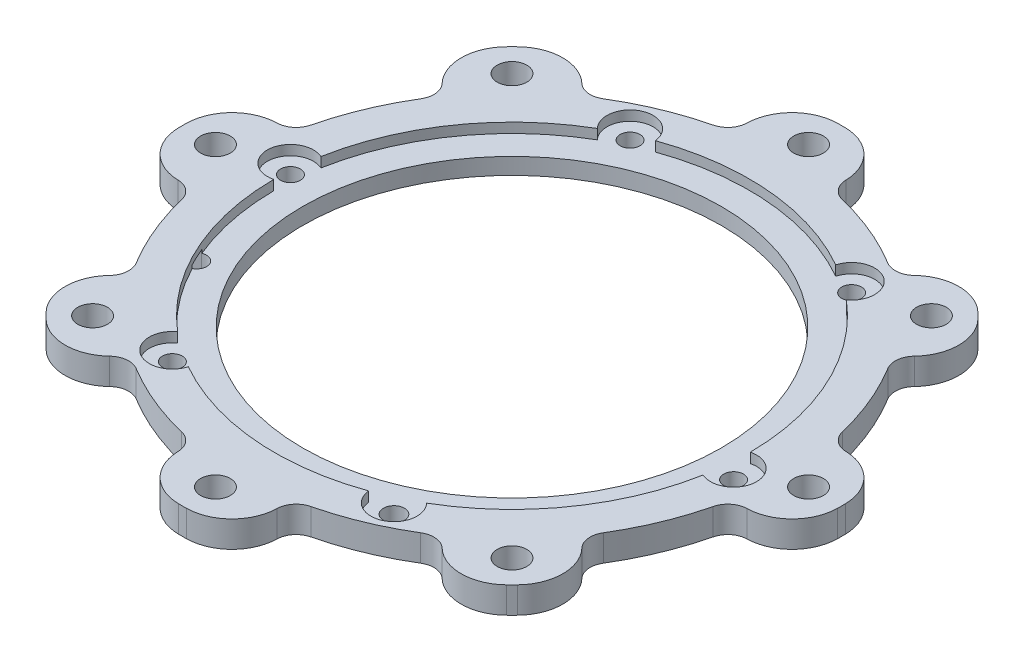
SolidWorks part; units mm, degrees
material "7075-T6 (SN)"
ref_plane "Front Plane" through (0, 0, 0) normal (0, 0, 1) x (1, 0, 0)
ref_plane "Top Plane" through (0, 0, 0) normal (0, 1, 0) x (1, 0, 0)
ref_plane "Right Plane" through (0, 0, 0) normal (1, 0, 0) x (0, 0, -1)
sketch "Sketch1" plane through (0, 0, 0) normal (0, 1, 0) x (1, 0, 0)
  circle A0 centre (0, 0) radius 50
  circle A1 centre (0, 0) radius 30
  dimension "D1" = 100
  dimension "D2" = 60
extrude "Boss-Extrude1" add sketch "Sketch1" along normal blind 4
sketch "Sketch2" plane through (0, 4, 0) normal (0, 1, 0) x (1, 0, 0)
  circle A0 centre (0, 0) radius 39
  circle A1 centre (0, 0) radius 30
  circle A2 centre (0, 0) radius 30 construction
  dimension "D1" = 78
extrude "Boss-Extrude2" add sketch "Sketch2" along normal blind 1
sketch "Sketch3" plane through (0, 0, 0) normal (0, -1, 0) x (1, 0, 0)
  circle A0 centre (0, 0) radius 31.75
  dimension "D1" = 63.5
extrude "Cut-Extrude1" cut sketch "Sketch3" against normal blind 1
sketch "Sketch4" plane through (0, 0, 0) normal (0, -1, 0) x (1, 0, 0)
  line L0 (0, 0) -> (50000, 0) construction
  line L1 (0, 0) -> (0, 50000) construction
  circle A0 centre (0, 0) radius 45 construction
  circle A1 centre (0, 45) radius 2.25
  dimension "D1" = 90
  dimension "D2" = 4.5
extrude "Cut-Extrude2" cut sketch "Sketch4" against normal blind 10
pattern_circular "CirPattern1" count 8 over 360 about axis through (0, 0, 0) along (0, 1, 0) of "Cut-Extrude2"
sketch "Sketch5" plane through (0, 0, 0) normal (0, -1, 0) x (1, 0, 0)
  circle A0 centre (0, 0) radius 31.75 construction
  circle A1 centre (0, 0) radius 31.75
extrude "Cut-Extrude3" cut sketch "Sketch5" against normal blind 27
sketch "Sketch6" plane through (0, 5, 0) normal (0, 1, 0) x (1, 0, 0)
  line L0 (0, 0) -> (49808.2107, -4375.1737) construction
  line L1 (0, 50) -> (0, -49950) construction
  line L2 (0, 0) -> (-50000, 0) construction
  circle A0 centre (0, 0) radius 37 construction
  circle A1 centre (36.8581, -3.2376) radius 3.5
  dimension "D1" = 74
  dimension "D2" = 7
  dimension "D3" = 84.98
extrude "Cut-Extrude4" cut sketch "Sketch6" against normal blind 2.5
pattern_circular "CirPattern2" count 6 over 360 about axis through (0, 0, 0) along (0, 1, 0) of "Cut-Extrude4"
sketch "Sketch7" plane through (0, 5, 0) normal (0, 1, 0) x (1, 0, 0)
  circle A0 centre (-21.2329, -30.3012) radius 1.5
  circle A1 centre (15.6252, -33.5388) radius 1.5978
  circle A2 centre (36.8581, -3.2376) radius 1.5
  circle A3 centre (21.2329, 30.3012) radius 1.5
  circle A4 centre (-15.6252, 33.5388) radius 1.5
  circle A5 centre (-36.8581, 3.2376) radius 1.5
  dimension "D1" = 3
extrude "Cut-Extrude5" cut sketch "Sketch7" against normal blind 15
sketch "Sketch8" plane through (0, 0, 0) normal (0, -1, 0) x (1, 0, 0)
  line L0 (0, 0) -> (50000, 0) construction
  line L1 (0, 0) -> (0, 50000) construction
  line L2 (0, 0) -> (20734.6621, -45498.0635) construction
  line L3 (0, 0) -> (35355.3391, -35355.3391) construction
  line L4 (7.5, -40.8167) -> (7.5, -49.4343)
  line L5 (23.5584, -34.165) -> (29.652, -40.2586)
  circle A2 centre (0, 0) radius 50 construction
  arc A3 (7.5, -40.8167) -> (23.5584, -34.165) centre (0, 0) ccw
  arc A4 (7.5, -49.4343) -> (29.652, -40.2586) centre (0, 0) ccw
  dimension "D4" = 41.5
  dimension "D1" = 24.5
  dimension "D2" = 15
  dimension "D3" = 15
extrude "Cut-Extrude6" cut sketch "Sketch8" against normal blind 13
pattern_circular "CirPattern3" count 8 over 360 about axis through (0, 0, 0) along (0, 1, 0) of "Cut-Extrude6"
fillet "Fillet1" radius 3 16 edges at (-7.5, 2, -40.8167) (-23.5584, 2, -34.165) (-34.165, 2, -23.5584) (-40.8167, 2, -7.5) (-40.8167, 2, 7.5) (-34.165, 2, 23.5584) (-23.5584, 2, 34.165) (-7.5, 2, 40.8167) (7.5, 2, 40.8167) (23.5584, 2, 34.165) (34.165, 2, 23.5584) (40.8167, 2, 7.5) (40.8167, 2, -7.5) (34.165, 2, -23.5584) (23.5584, 2, -34.165) (7.5, 2, -40.8167)
sketch "Sketch9" plane through (0, 5, 0) normal (0, 1, 0) x (1, 0, 0)
  circle A0 centre (0, 0) radius 36
  dimension "D1" = 72
extrude "Cut-Extrude7" cut sketch "Sketch9" against normal up to surface (2.5 mm away) up to face at (-15.6252, 2.5, -32.0388)
fillet "Fillet2" radius 7 16 edges at (40.2586, 2, -29.652) (29.652, 2, -40.2586) (7.5, 2, -49.4343) (-7.5, 2, -49.4343) (-29.652, 2, -40.2586) (-40.2586, 2, -29.652) (-49.4343, 2, -7.5) (-49.4343, 2, 7.5) (-40.2586, 2, 29.652) (-29.652, 2, 40.2586) (-7.5, 2, 49.4343) (7.5, 2, 49.4343) (29.652, 2, 40.2586) (40.2586, 2, 29.652) (49.4343, 2, 7.5) (49.4343, 2, -7.5)
sketch "Sketch10" plane through (0, 5, 0) normal (0, 1, 0) x (1, 0, 0)
  circle A0 centre (0, 0) radius 50
  dimension "D1" = 100
extrude "Cut-Extrude8" cut sketch "Sketch10" against normal up to surface (1 mm away) up to face at (0, 4, 0)
sketch "Sketch12" plane through (0, 0, 0) normal (0, -1, 0) x (1, 0, 0)
  line L0 (0, 0) -> (50000, 0) construction
  line L1 (0, 0) -> (-45322.7627, 21115.0937) construction
  line L2 (-36.8581, -3.2376) -> (49771.3526, 4371.9361) construction
  circle A0 centre (0, 0) radius 37 construction
  circle A1 centre (-33.5388, 15.6252) radius 1.5
  circle A2 centre (33.5388, -15.6252) radius 1.5
  dimension "D2" = 3
  dimension "D1" = 30
extrude "Cut-Extrude9" cut sketch "Sketch12" against normal blind 3
sketch "Sketch13" plane through (0, 0, 0) normal (0, -1, 0) x (1, 0, 0)
  line L0 (-33.5388, 15.6252) -> (45289.2238, -21099.4686) construction
  line L1 (0, 0) -> (-21115.0937, -45322.7627) construction
  line L2 (-32.6324, 15.2029) -> (-34.4453, 16.0475) construction
  line L3 (-33.2658, 13.8432) -> (-35.0788, 14.6878)
  line L4 (-31.9989, 16.5626) -> (-33.8118, 17.4072)
  arc A1 (-33.2658, 13.8432) -> (-31.9989, 16.5626) centre (-32.6324, 15.2029) ccw
  arc A2 (-33.8118, 17.4072) -> (-35.0788, 14.6878) centre (-34.4453, 16.0475) ccw
  circle A3 centre (-33.5388, 15.6252) radius 1.5 construction
  point P9 (-33.5388, 15.6252)
  dimension "D1" = 2
extrude "Cut-Extrude10" cut sketch "Sketch13" against normal up to surface (3 mm away) up to face at (-33.7655, 3, 15.7307)
